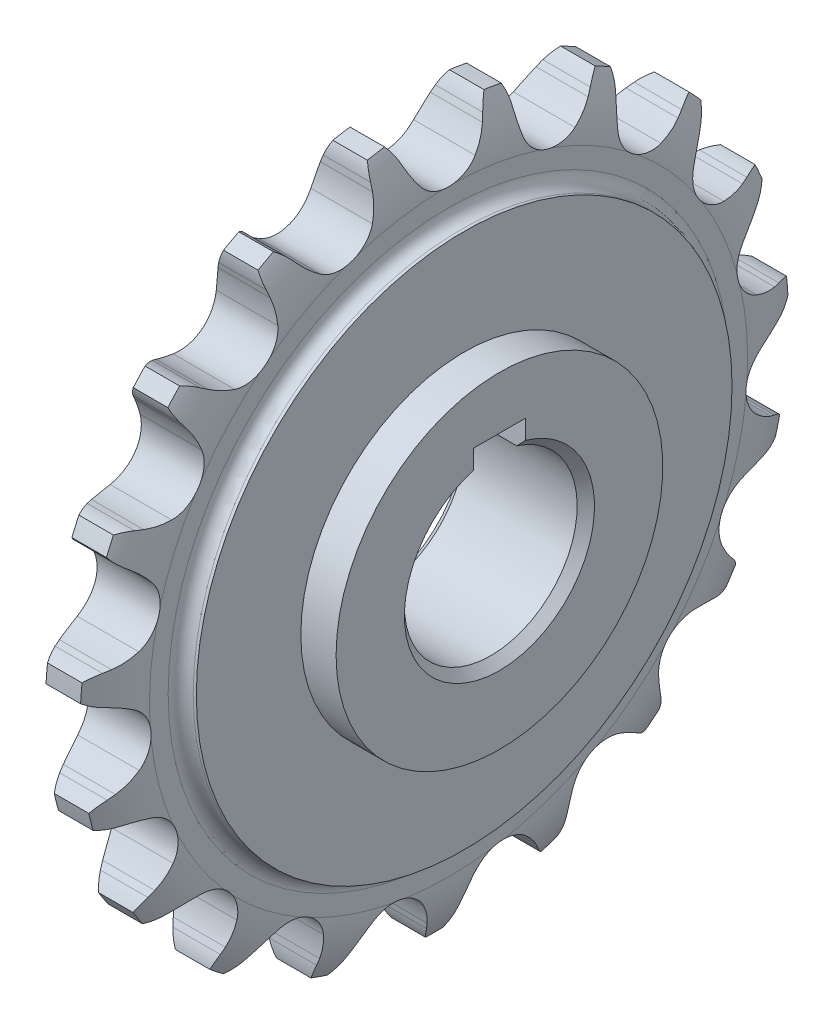
from build123d import *

# Parameters (mm, degrees)
CUT_EXTRUDE_1_DEPTH      = 5.460069882
PATTERN_CIRCULAR_1_COUNT = 19
SKETCH_3_W               = 4.079860236
SKETCH_3_H               = 8.904926129
SKETCH_4_W               = 6
SKETCH_4_H               = 3.260607938
CUT_EXTRUDE_2_DEPTH      = 60.844303841
CHAMFER_1_SIZE           = 1
CHAMFER_3_SIZE           = 1


with BuildPart() as part:
    # 草图1 → 旋转1 (revolve)
    with BuildSketch(Plane.XY, mode=Mode.PRIVATE) as revolve_1_sk:
        with BuildLine():
            Line((-5.460069882, 10), (-5.460069882, 31))
            Line((-5.460069882, 31), (-5.098105905, 31))
            ThreePointArc((-5.098105905, 31), (-4.074317176, 31.424067176), (-3.65025, 32.447855905))
            Line((-3.65025, 32.447855905), (-3.65025, 34.619639763))
            ThreePointArc((-3.65025, 34.619639763), (-3.245836945, 37.918781526), (-1.99925, 41))
            Line((-1.99925, 41), (1.99925, 41))
            ThreePointArc((1.99925, 41), (3.245836945, 37.918781526), (3.65025, 34.619639763))
            Line((3.65025, 34.619639763), (3.65025, 32.447855905))
            ThreePointArc((3.65025, 32.447855905), (4.074317176, 31.424067176), (5.098105905, 31))
            Line((5.098105905, 31), (5.460069882, 31))
            Line((5.460069882, 31), (5.460069882, 10))
            Line((5.460069882, 10), (-5.460069882, 10))
        make_face()
    revolve(revolve_1_sk.sketch.rotate(Axis((-6.35, 0, 0), (1, 0, 0)), 90), axis=Axis((-6.35, 0, 0), (1, 0, 0)))

    # 草图2 → 切除-拉伸1 (cut, symmetric)
    with BuildSketch(Plane(origin=(0, 0, 0), x_dir=(0, 0, -1), z_dir=(1, 0, 0))):
        with BuildLine():
            Line((4.552244709, 38.426451297), (4.858741585, 39.1448403))
            ThreePointArc((4.858741585, 39.1448403), (5.250930322, 39.90290393), (5.750855114, 40.594675334))
            ThreePointArc((5.750855114, 40.594675334), (0, 41), (-5.750855114, 40.594675334))
            ThreePointArc((-5.750855114, 40.594675334), (-5.250930322, 39.90290393), (-4.858741585, 39.1448403))
            Line((-4.858741585, 39.1448403), (-4.552244709, 38.426451297))
            ThreePointArc((-4.552244709, 38.426451297), (-3.937302758, 37.212676935), (-3.168676608, 36.089905522))
            ThreePointArc((-3.168676608, 36.089905522), (0, 34.549839763), (3.168676608, 36.089905522))
            ThreePointArc((3.168676608, 36.089905522), (3.937302758, 37.212676935), (4.552244709, 38.426451297))
        make_face()
    cut_extrude_1 = extrude(amount=CUT_EXTRUDE_1_DEPTH, both=True, mode=Mode.SUBTRACT)

    # 阵列(圆周)1: 切除-拉伸1 ×19 about axis
    pattern_circular_1_axis = Axis((0, 0, 0), (1, 0, 0))
    for i in range(1, PATTERN_CIRCULAR_1_COUNT):
        add(cut_extrude_1.rotate(pattern_circular_1_axis, i * 360 / PATTERN_CIRCULAR_1_COUNT), mode=Mode.SUBTRACT)

    # 草图3 → 旋转2 (revolve)
    with BuildSketch(Plane.XY, mode=Mode.PRIVATE) as revolve_2_sk:
        with Locations((7.5, 14.452463064)):
            Rectangle(SKETCH_3_W, SKETCH_3_H)
    revolve(revolve_2_sk.sketch.rotate(Axis((0, 0, 0), (1, 0, 0)), 90), axis=Axis((0, 0, 0), (1, 0, 0)))

    # 草图4 → 切除-拉伸2 (cut, through all)
    with BuildSketch(Plane.ZY.offset(5.460069882)):
        with Locations((0, 11.169695983)):
            Rectangle(SKETCH_4_W, SKETCH_4_H)
    extrude(amount=-CUT_EXTRUDE_2_DEPTH, mode=Mode.SUBTRACT)

    # 倒角1
    chamfer_1_edges = [part.edges().sort_by_distance(p)[0] for p in [
        (-5.460069882, -10, 0),
    ]]
    chamfer(chamfer_1_edges, length=CHAMFER_1_SIZE)

    # 倒角3
    chamfer_3_edges = [part.edges().sort_by_distance(p)[0] for p in [
        (9.539930118, -10, 0),
    ]]
    chamfer(chamfer_3_edges, length=CHAMFER_3_SIZE)


solid = part.part
